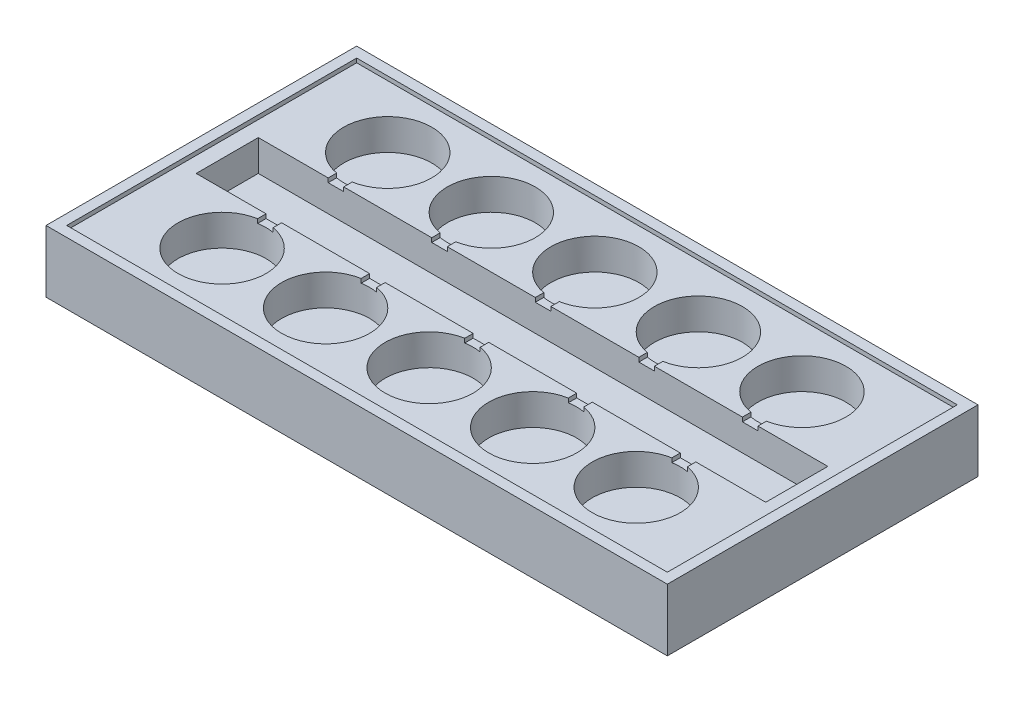
SolidWorks part; units mm, degrees
ref_plane "Front Plane" through (0, 0, 0) normal (0, 0, 1) x (1, 0, 0)
ref_plane "Top Plane" through (0, 0, 0) normal (0, 1, 0) x (1, 0, 0)
ref_plane "Right Plane" through (0, 0, 0) normal (1, 0, 0) x (0, 0, -1)
sketch "Sketch1" plane through (0, 0, 0) normal (0, 1, 0) x (1, 0, 0)
  line L1 (-300, 150) -> (300, 150)
  line L2 (-300, 150) -> (-300, -150)
  line L3 (-300, -150) -> (300, -150)
  line L4 (300, 150) -> (300, -150)
  line L5 (-300, 150) -> (300, -150) construction
  line L6 (-300, -150) -> (300, 150) construction
  point P0 (0, 0)
  dimension "D1" = 600
  dimension "D2" = 300
extrude "Boss-Extrude1" add sketch "Sketch1" along normal blind 60
sketch "Sketch2" plane through (0, 60, 0) normal (0, 1, 0) x (1, 0, 0)
  line L0 (0, 0) -> (0, 130.681) construction
  line L1 (0, 0) -> (214.7524, 0) construction
  line L3 (-275, 30) -> (275, 30)
  line L4 (-275, 30) -> (-275, -30)
  line L5 (-275, -30) -> (275, -30)
  line L6 (275, 30) -> (275, -30)
  line L7 (-275, 30) -> (275, -30) construction
  line L8 (-275, -30) -> (275, 30) construction
  circle A0 centre (0, 80) radius 42.5
  circle A1 centre (0, -80) radius 42.5
  circle A2 centre (-100, 80) radius 42.5
  circle A3 centre (-200, 80) radius 42.5
  circle A4 centre (200, 80) radius 42.5
  circle A5 centre (100, 80) radius 42.5
  circle A6 centre (200, -80) radius 42.5
  circle A7 centre (100, -80) radius 42.5
  circle A8 centre (-100, -80) radius 42.5
  circle A9 centre (-200, -80) radius 42.5
  point P4 (0, 0)
  dimension "D3" = 85
  dimension "D4" = 50
  dimension "D5" = 200
  dimension "D1" = 60
  dimension "D2" = 550
  dimension "D6" = 100
extrude "Cut-Extrude1" cut sketch "Sketch2" against normal blind 34
sketch "Sketch3" plane through (0, 60, 0) normal (0, 1, 0) x (1, 0, 0)
  line L0 (300, 150) -> (-300, 150) construction
  line L1 (-290, 140) -> (290, 140)
  line L2 (-290, 140) -> (-290, -140)
  line L3 (-290, -140) -> (290, -140)
  line L4 (290, 140) -> (290, -140)
  line L5 (-290, 140) -> (290, -140) construction
  line L6 (-290, -140) -> (290, 140) construction
  line L7 (-300, 150) -> (-300, -150) construction
  point P0 (0, 0)
  dimension "D1" = 10
  dimension "D2" = 10
extrude "Cut-Extrude2" cut sketch "Sketch3" against normal blind 4
sketch "Sketch4" plane through (0, 56, 0) normal (0, 1, 0) x (1, 0, 0)
  line L1 (-7.5, 48.352) -> (7.5, 48.352)
  line L2 (-7.5, 48.352) -> (-7.5, -48.352)
  line L3 (-7.5, -48.352) -> (7.5, -48.352)
  line L4 (7.5, 48.352) -> (7.5, -48.352)
  line L5 (-7.5, 48.352) -> (7.5, -48.352) construction
  line L6 (-7.5, -48.352) -> (7.5, 48.352) construction
  point P0 (0, 0)
  dimension "D1" = 15
extrude "Cut-Extrude3" cut sketch "Sketch4" against normal blind 4
pattern_linear "LPattern1" count 3 spacing 100 along (-1, 0, 0) count 3 spacing 100 along (1, 0, 0) seed only of "Cut-Extrude3"
